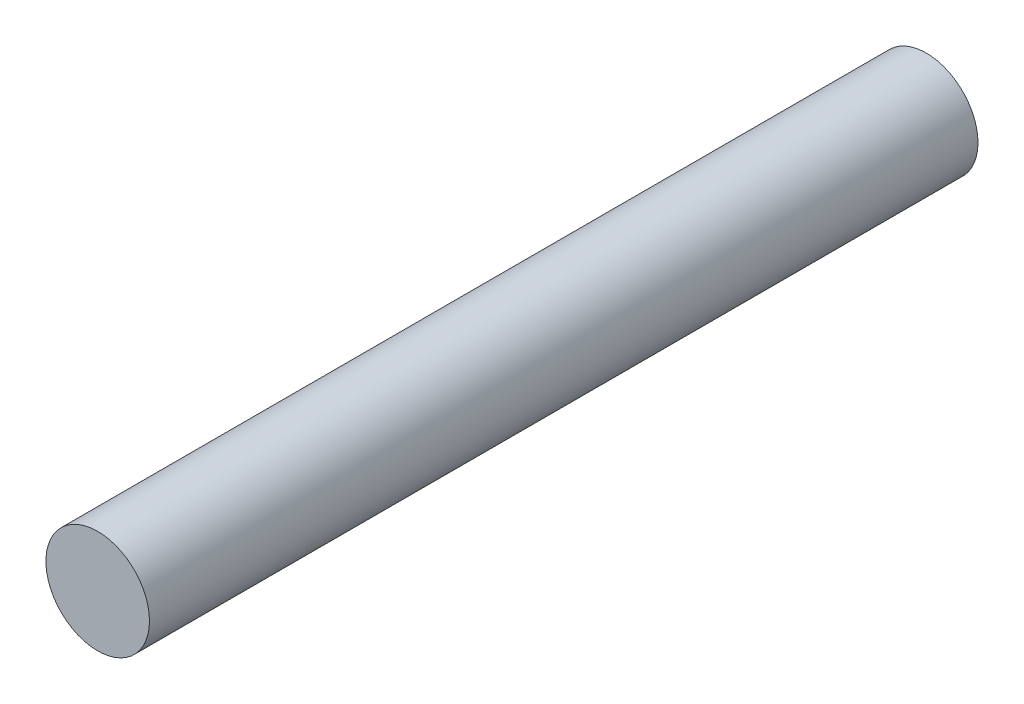
from build123d import *

# Parameters (mm, degrees)
BOSS_EXTRUDE1_DEPTH      = 200
BOSS_EXTRUDE1_DEPTH_BACK = 40
SKETCH2_R                = 15


with BuildPart() as part:
    # Sketch2 → Boss-Extrude1 (new, two sides: drawn at the far end of the back side and taken through both)
    with BuildSketch(Plane.XY.offset(-BOSS_EXTRUDE1_DEPTH_BACK)):
        Circle(SKETCH2_R)
    extrude(amount=BOSS_EXTRUDE1_DEPTH + BOSS_EXTRUDE1_DEPTH_BACK)


solid = part.part
